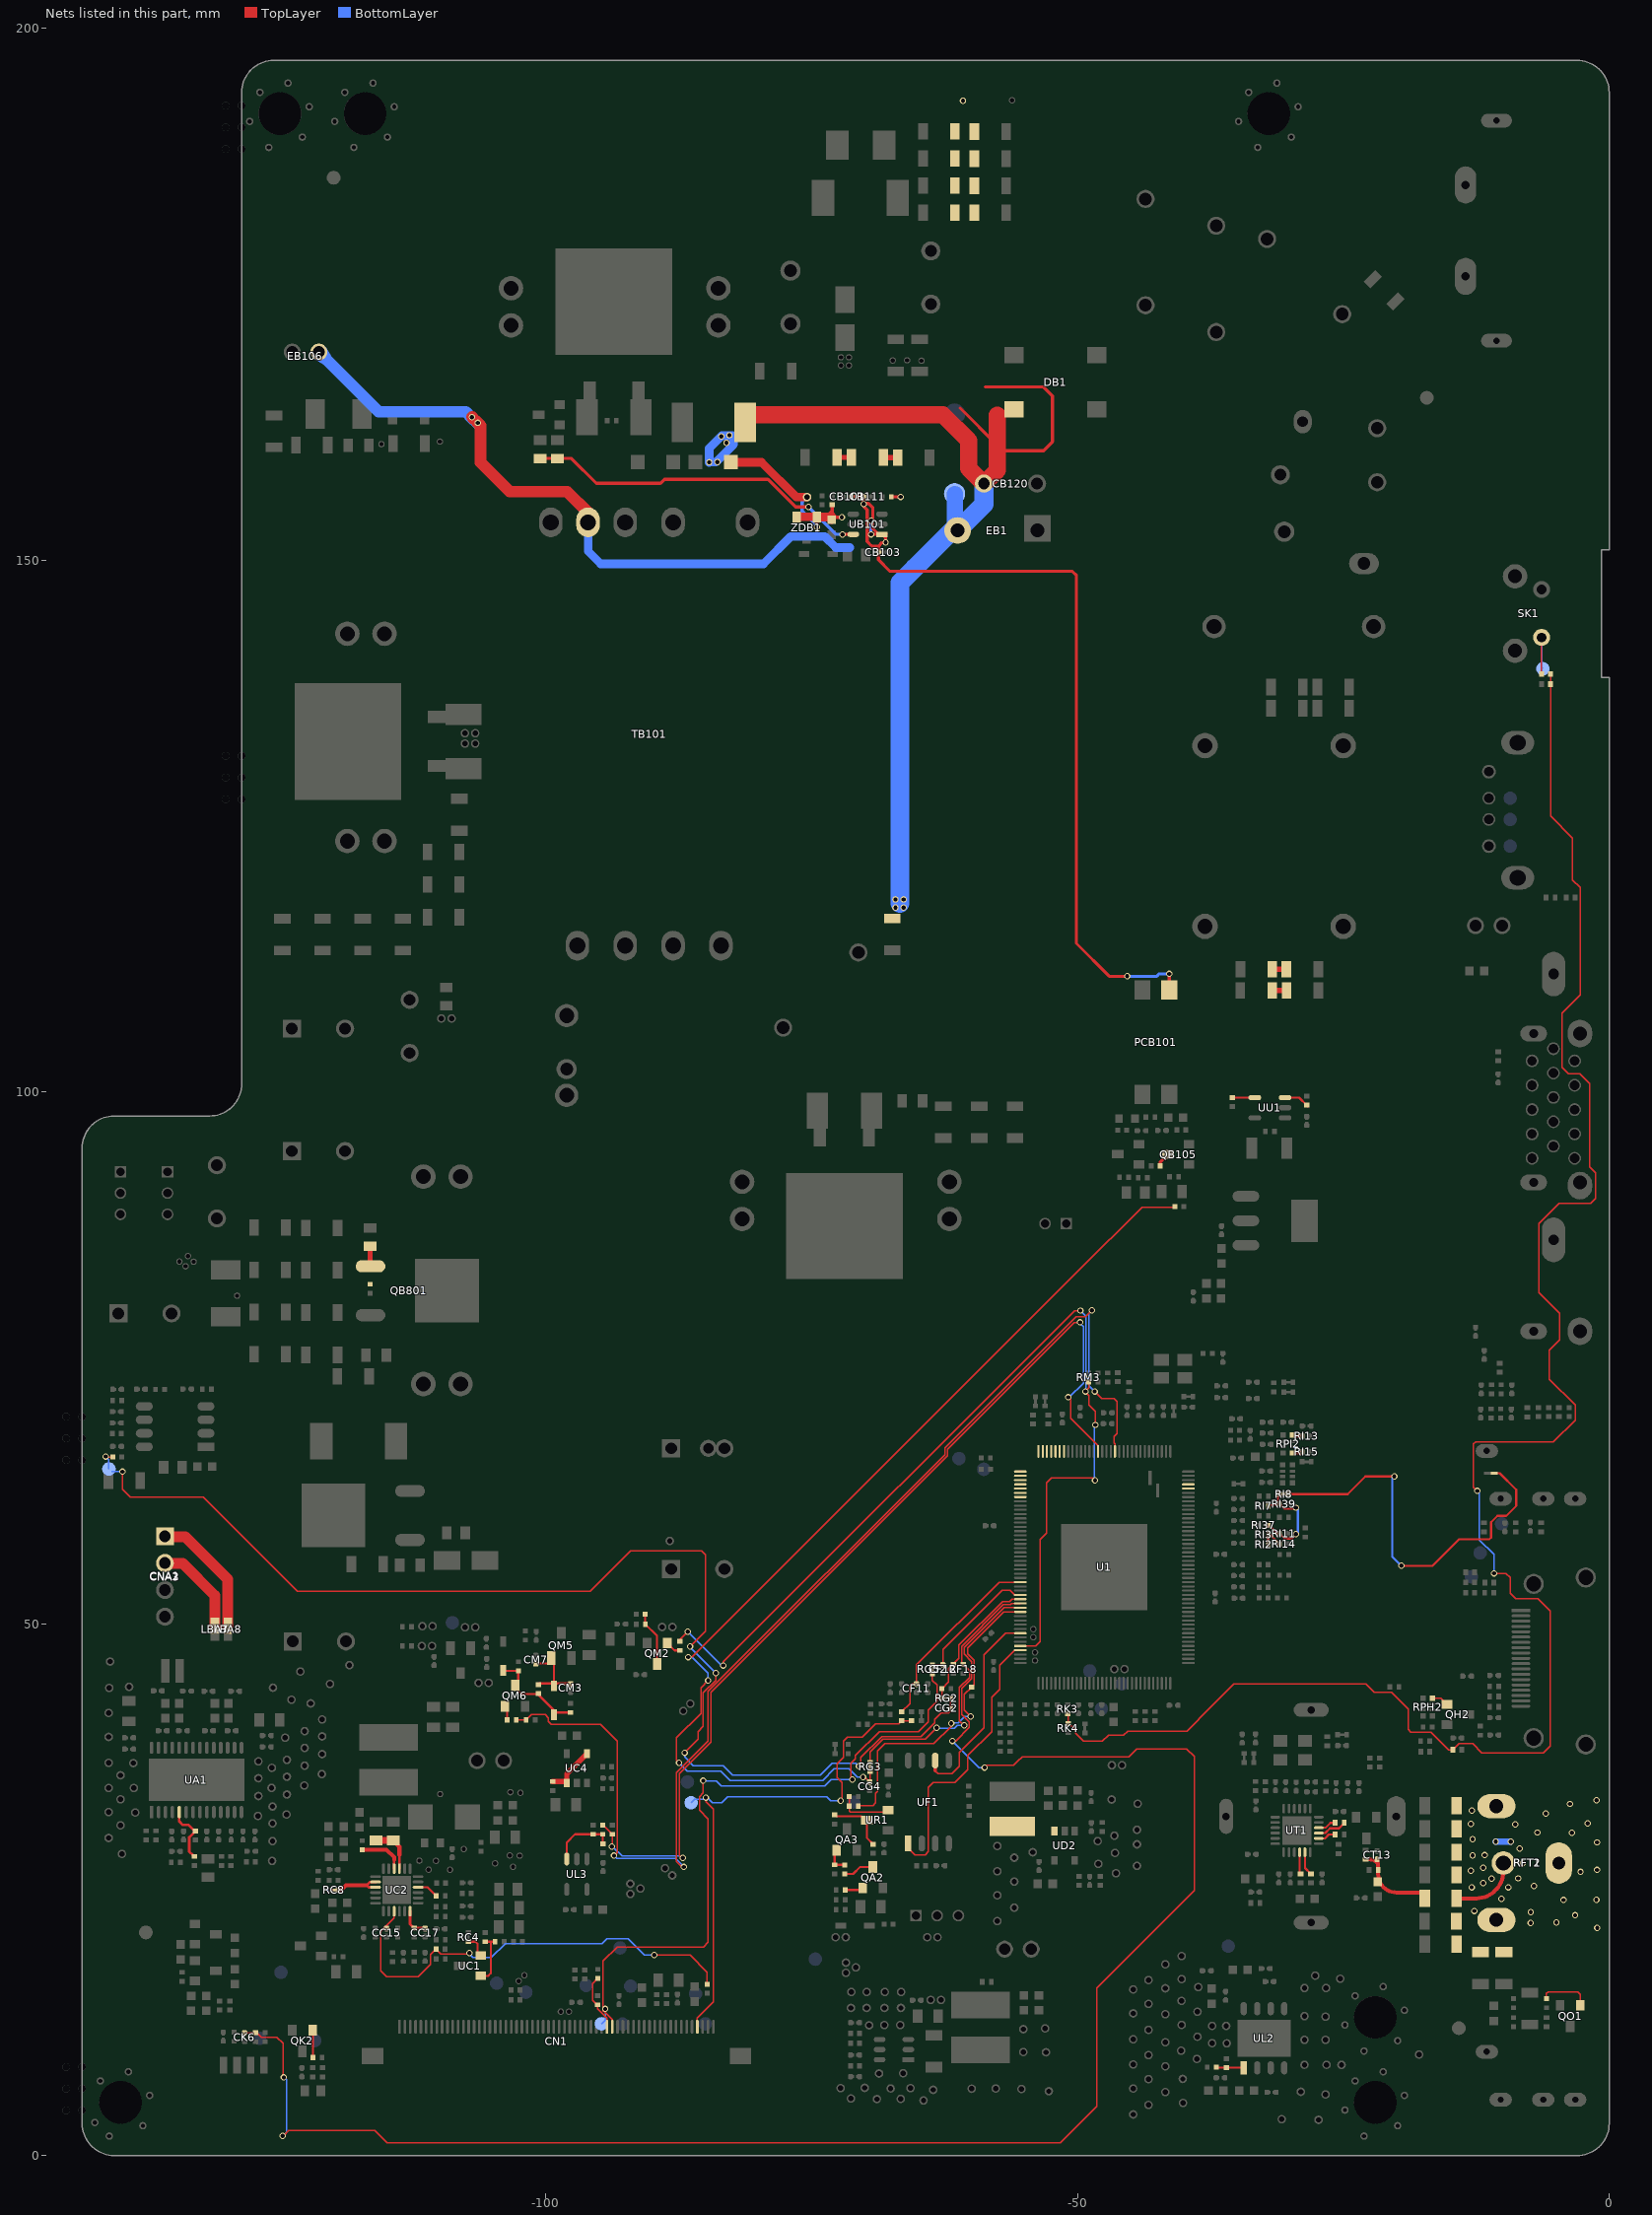
[diagram p0: the nets of this part, all layers, seen from the top]
# Altium PCB MISC86383-9.PcbDoc (part 14 of 18)
Units mm, origin at the board's own origin, x right, y up, seen from the top; angles counter-clockwise.
Board outline 143.6 x 197 mm, 2 copper layers (TopLayer, BottomLayer), stack 1.571 mm thick; 743 components, 401 nets, 2996 pads, 1077 vias.
Unrouted connection lines stored in the file: 4.

## Via types
v1: diameter 0.6, hole 0.4, TopLayer to BottomLayer, tented both sides, 993 vias
v2: diameter 0.6, hole 0.4, TopLayer to BottomLayer, 65 vias
v3: diameter 0.7, hole 0.5, TopLayer to BottomLayer, tented both sides, 15 vias
v4: diameter 0.8, hole 0.5, TopLayer to BottomLayer, tented both sides, 4 vias

## Nets (pads, with @x,y where several pads share a name; then routed paths per layer and width w, separated by ;. In a path a pad name is that pad's centre, name@x,y a point inside that pad or via, vN(x,y) a via of type N, cw(c..) or ccw(c..) an arc to the next point about the centre after c; other vN are vias at no path point) (continued)
NetDK1_K: DK1.K DK2.K RK3.2 RK4.1 RK6.1 | length 177.8
  TopLayer w0.127: RK3.2@-50.862,41.54 -50.862,40.625 RK4.1@-50.874,40.612 -50.779,40.612 -50.189,40.022 -50.189,39.704 -49.439,38.955 -47.656,38.955 -47.092,39.519 -45.657,39.519 -45.281,39.895 -39.723,39.895 -37.47,42.149 -37.47,42.171 -35.277,44.364 -22.893,44.364 -22.069,43.539 -20.456,43.539 -18.91,41.993 -18.91,40.058 -18.676,39.825 -16.762,39.825 -15.088,38.151 DK2.K@-14.7,38.151 -14.13,38.721 -12.813,38.721 -11.969,37.877 -6.175,37.877 -5.537,38.515 -5.537,51.225 -6.687,52.375 -8.81,52.375 -9.301,52.866 -9.301,54.333 -9.708,54.74 v1(-10.825,54.74) ; v1(-12.408,62.497) -12.75,62.839 -12.75,66.897 -12.56,67.087 -5.265,67.087 -3.2,69.152 -3.2,70.561 -5.625,72.986 -5.625,75.732 -4.674,76.683 -4.674,79.18 -6.617,81.123 -6.617,87.624 -4.705,89.535 -1.753,89.535 -1.295,89.992 -1.295,92.411 -1.829,92.945 -1.829,100.787 -2.743,101.702 -3.835,101.702 -4.445,102.311 -4.445,107.417 -2.729,109.132 -2.729,119.219 -3.437,119.927 -3.437,123.888 -5.519,125.969 DK1.K@-5.519,138.354 RK6.1@-5.519,139.294
  BottomLayer w0.127: v1(-12.408,62.497) -12.197,62.286 -12.197,57.897 -10.825,56.525 v1(-10.825,54.74)
NetKEY_1: KEY.1 RK6.2 SK1.2 | length 6.5
  TopLayer w0.127: RK6.2@-6.369,139.294 -6.369,142.731 SK1.2@-6.35,142.75
  BottomLayer w0.127: SK1.2@-6.35,142.75 -6.35,139.916 KEY.1@-6.236,139.802
NetLD2_2: LD2.2 UD2.3
NetLT1_2: LT1.2 UT1.23 | length 2.3
  TopLayer w0.203: UT1.23@-28.61,28.52 -28.61,27.033 LT1.2@-28.064,26.487
NetLT2_1: LT2.1 UT1.22 | length 2
  TopLayer w0.203: LT2.1@-29.11,26.568 UT1.22@-29.11,28.52
NetLT8_1: LT8.1 UT1.2 | length 1.7
  TopLayer w0.203: UT1.2@-27.31,29.82 -26.732,29.82 -26.376,30.177 LT8.1@-25.771,30.177
NetLT10_1: LT10.1 UT1.4 | length 1.7
  TopLayer w0.203: UT1.4@-27.31,30.82 -26.669,30.82 -26.208,31.282 LT10.1@-25.771,31.282
NetLT10_2: LT10.2 UT1.3 | length 2.8
  TopLayer w0.203: UT1.3@-27.31,30.32 -26.702,30.32 -26.261,30.761 -25.41,30.761 -24.921,31.25 LT10.2@-24.921,31.282
NetQA2_B: QA2.B RA19.1 | length 1.7
  TopLayer w0.203: RA19.1@-71.855,24.98 -70.388,24.98 QA2.B@-70.21,25.157
NetQA2_C: QA2.C RA10.1 | length 2.9
  TopLayer w0.203: RA10.1@-71.89,26.472 -71.096,26.472 -70.428,27.139 QA2.C@-69.245,27.139
NetQA3_B: QA3.B RA10.2 RA38.2 | length 2.4
  TopLayer w0.203: QA3.B@-72.649,28.713 -72.83,28.532 RA38.2@-72.83,27.334 -71.903,27.334 RA10.2@-71.89,27.322
NetQB105_C: QB105.C RB180.1 | length 1.4
  TopLayer w0.3: RB180.1@-42.222,93.066 -42.222,93.428 QB105.C@-41.504,94.145
NetQB801_G: QB801.G RB807.2 RB808.2 | length 1.9
  TopLayer w0.5: RB807.2@-116.523,85.494 -116.523,83.657 QB801.G@-116.484,83.618
NetQH2_B: QH2.B RPH2.7 | length 1.6
  TopLayer w0.127: RPH2.7@-16.606,43.014 -15.832,43.014 QH2.B@-15.241,42.423
NetQK2_B: QK2.B RK20.1 | length 2.6
  TopLayer w0.203: QK2.B@-121.933,11.786 -121.888,11.741 RK20.1@-121.888,9.195
NetQM2_B: QM2.B RM4.1 | length 1.7
  TopLayer w0.203: QM2.B@-88.424,48.342 QM2.B@-88.57,48.197 -88.57,48.171 -87.891,47.492 RM4.1@-87.376,47.492
NetQM2_C: QM2.C RM1.1 RM2.1 | length 5.1
  TopLayer w0.203: RM1.1@-90.647,50.902 -90.647,49.975 RM2.1@-90.634,49.962 -89.535,48.863 QM2.C@-89.535,46.215
NetQM6_B: QM6.B RM8.2 | length 1.4
  TopLayer w0.203: QM6.B@-103.848,42.228 -103.625,42.005 RM8.2@-103.625,40.957
NetQO1_B: QO1.B RO10.1 | length 4.9
  TopLayer w0.127: RO10.1@-5.893,14.746 -5.893,15.24 -5.74,15.392 -2.946,15.392 -2.705,15.151 QO1.B@-2.705,14.118
NetRA4_1: RA4.1 RA14.2 UA1.5 | length 5.6
  TopLayer w0.254: UA1.5@-134.47,32.291 -134.47,31.411 -134.14,31.08 -133.592,31.08 -133.02,30.509 RA14.2@-132.947,30.509 -133.53,29.925 -133.53,28.58 -133.173,28.223 -133.048,28.223 RA4.1@-133.004,28.223
NetRB101_2: RB101.2 RB102.1 | length 1.3
  TopLayer w0.5: RB102.1@-31.685,109.563 RB101.2@-30.342,109.563
NetRB106_1: RB106.1 RB107.1 UB101.6 | length 32.7
  TopLayer w0.3: RB107.1@-100.546,159.56 -100.533,159.573 RB106.1@-98.92,159.573 -97.584,159.573 -95.25,157.239 -89.217,157.239 -88.836,157.62 -79.111,157.62 -76.508,155.016 v2(-75.286,155.016) ; v2(-72.098,152.438) -72.095,152.441 UB101.6@-71.086,152.441
  BottomLayer w0.3: v2(-75.286,155.016) -72.707,152.438 v2(-72.098,152.438)
NetRB141_1: RB141.1 RB142.2 | length 1.9
  TopLayer w0.3: RB142.2@-31.672,111.544 -31.067,111.544
  TopLayer w0.5: RB142.2@-31.672,111.544 -31.66,111.557 RB141.1@-30.354,111.557
NetRB143_1: RB143.1 RB144.2 | length 1.3
  TopLayer w0.5: RB144.2@-68.261,159.677 -68.248,159.664 RB143.1@-66.918,159.664
NetRB144_1: RB144.1 RB145.2 | length 1.4
  TopLayer w0.5: RB145.2@-72.617,159.677 RB144.1@-71.261,159.677
NetRB150_1: pad.VIA5@-60.769,193.218 RB150.1 RB151.1 RB152.1 RB153.2 RB154.2 RB155.2 RB156.1 RB157.2
NetRC2_1: RC2.1 RC3.2 UC1.1 | length 4.9
  TopLayer w0.203: UC1.1@-106.121,16.891 -105.41,16.891 -105.177,17.124 -105.177,20.013 ; RC3.2@-105.715,20.098 -104.787,20.098 RC2.1@-104.768,20.117
NetRC4_1: RC4.1 UC1.2 | length 2.2
  TopLayer w0.203: RC4.1@-107.29,20.098 -106.611,20.098 -106.426,19.914 -106.426,19.05 -106.172,18.796 UC1.2@-106.121,18.796
NetRC8_2: RC8.2 RC8.3 UC2.2 UC2.3 | length 4.7
  TopLayer w0.254: UC2.3@-116.014,25.223 -116.638,25.223 -116.827,25.413 -116.517,25.723 UC2.2@-116.014,25.723
  TopLayer w0.381: RC8.2@-119.52,24.948 -119.269,24.948 -118.804,25.413 -116.827,25.413
NetRC13_1: RC13.1 UC2.16 | length 2
  TopLayer w0.203: UC2.16@-112.014,25.223 -111.131,25.223 RC13.1@-110.309,24.401
NetRC36_1: RC36.1 UC4.1 UC4.4 | length 4.9
  TopLayer w0.508: RC36.1@-99.365,35.172 -98.165,35.172 UC4.1@-98.029,35.036 -98.029,35.886 UC4.4@-96.129,37.786
NetRG6_1: RG6.1 UC2.22 | length 4.4
  TopLayer w0.254: UC2.22@-114.264,26.973 -114.264,27.813
  TopLayer w0.381: RG6.1@-117.259,28.76 -114.98,28.76 -114.264,28.044 -114.264,27.813
NetRG58_1: RG58.1 RG63.1 UC2.21 | length 4.5
  TopLayer w0.254: UC2.21@-113.764,26.973 -113.764,28.27
  TopLayer w0.381: RG63.1@-114.351,29.627 -113.764,29.04 -113.764,28.27
  TopLayer w0.61: RG58.1@-115.976,29.627 RG63.1@-114.351,29.627
NetRI2_1: RI2.1 RI3.2 RI14.2 | length 2.3
  TopLayer w0.178: RI14.2@-30.991,57.495 RI14.2@-30.989,57.497
  TopLayer w0.203: RI2.1@-32.057,57.483 RI3.2@-32.057,58.372 -31.867,58.372 RI14.2@-30.991,57.495
NetRI7_2: RI7.2 RI8.1 RI11.2 RI37.2 RI39.2 | length 9.7
  TopLayer w0.178: RI7.2@-32.057,61.077 -31.968,61.166 RI39.2@-31.015,61.166 ; RI8.1@-31.015,62.194 -31.136,62.074 -31.136,61.414 RI39.2@-31.002,61.28 -30.995,61.28 -30.529,60.814 v1@-29.57,60.814
  TopLayer w0.203: RI37.2@-32.057,59.248 -31.974,59.248 -31.136,58.41 RI11.2@-31.002,58.41 ; RI11.2@-31.002,58.486 -30.523,58.007 -29.832,58.007 -29.472,58.368 v1(-29.472,58.422)
  BottomLayer w0.203: v1(-29.472,58.422) -29.274,58.621 -29.274,60.713 v1(-29.472,60.912)
NetRI8_2: RI8.2 RI8.3 RI10.JP_2K | length 37.7
  TopLayer w0.203: RI8.2@-30.165,62.194 -24.591,62.194 -22.935,63.851 v1(-20.206,63.851) ; v1(-19.553,55.452) -16.634,55.452 -14.149,57.937 -11.29,57.937 -11.112,58.115 -11.112,59.538 -10.506,60.144 -9.68,60.144 -8.737,61.087 -8.737,62.597 -10.3,64.16 RI10.JP_2K@-10.793,64.16
  BottomLayer w0.203: v1(-20.206,63.851) -20.404,63.652 -20.404,56.303 v1(-19.553,55.452)
NetRI13_2: RI13.2 RPI2.2 | length 1
  TopLayer w0.305: RPI2.2@-29.771,67.756 -29.671,67.655 RI13.2@-28.868,67.655 RI13.2@-28.907,67.616
NetRI15_2: RI15.2 RPI2.8 | length 1
  TopLayer w0.254: RPI2.8@-29.771,66.056 -28.994,66.056 RI15.2@-28.868,66.182
NetRL3_2: RL3.2 RL50.2 RL51.2 UL3.3 | length 6.2
  TopLayer w0.203: UL3.3@-98.016,27.879 -98.016,29.441 -97.25,30.207 RL3.2@-95.555,30.207 RL51.2@-94.64,30.207 -94.64,29.33 RL50.2@-94.628,29.318
NetRL4_2: RL4.2 RL5.1 UL2.1 | length 3.1
  TopLayer w0.203: RL5.1@-36.945,8.306 -36.901,8.262 RL4.2@-35.992,8.262 -34.387,8.262 UL2.1@-34.366,8.241 UL2.1@-34.366,7.849 ; UL2.1@-34.461,7.754 UL2.1@-34.385,7.83
NetRR5_1: RR5.1 RR6.1 UR1.3 | length 5.8
  TopLayer w0.203: RR6.1@-72.847,32.099 -72.809,32.061 -72.651,31.902 -70.333,31.902 -69.963,31.533 UR1.3@-69.792,31.533 -69.792,29.85 RR5.1@-69.207,29.265
NetRU4_1: RU4.1 UU1.4 | length 2.1
  TopLayer w0.203: RU4.1@-35.425,99.477 UU1.4@-33.327,99.477
NetRU45_1: RU45.1 UU1.3 | length 2.5
  TopLayer w0.203: UU1.3@-30.477,99.477 -29.164,99.477 -28.448,98.762 RU45.1@-28.346,98.66
OE1: CN1.57 OE1.1 RG40.2 RG46.2 | length 50.6
  TopLayer w0.127: CN1.57@-85.75,12.103 -85.75,12.923 -84.226,14.448 -84.226,32.564 -84.95,33.289 v1(-84.95,33.655) v1@-84.811,33.655 ; v1(-72.263,33.363) -72.128,33.498 -72.128,35.082 -72.606,35.56 -72.606,36.852 -72.005,37.453 -72.005,38.956 -71.642,39.319 -70.244,39.319 -68.982,40.581 -66.817,40.581 RG46.2@-66.523,40.875 RG40.2@-65.608,40.875
  BottomLayer w0.127: OE1.1@-86.335,33.172 -85.992,33.515 -85.09,33.515 v1(-84.95,33.655) ; v1@-84.811,33.655 -84.315,33.16 -83.455,33.16 -82.897,33.718 -73.566,33.718 -73.219,33.371 -72.271,33.371 v1(-72.263,33.363)
OE1/: CF11.1 RG46.1 U1.105 | length 18.2
  TopLayer w0.127: RG46.1@-66.523,41.725 -65.735,42.513 -65.735,44.145 -65.514,44.367 CF11.1@-65.151,44.367 -65.151,46.141 -57.379,53.913 U1.105@-55.371,53.913
PAIRMODE/: CN1.40 RG7.1 RG12.2 | length 5.4
  TopLayer w0.127: RG12.2@-95.123,14.174 RG12.2@-95.123,14.122 ; RG7.1@-95.11,16.656 -95.593,16.174 -95.593,14.592 -95.149,14.148 RG12.2@-95.123,14.122 ; CN1.40@-94.25,12.103 -94.25,12.916 -95.123,13.789 RG12.2@-95.123,14.122
PANEL5V_MOS_G: CM3.1 CM7.1 DM1.K QM5.G RM7.2 | length 7.3
  TopLayer w0.203: CM7.1@-100.94,46.197 -100.87,46.266 QM5.G@-99.682,46.266 ; RM7.2@-100.711,44.278 -100.602,44.388 DM1.K@-99.225,44.388 ; QM5.G@-99.49,46.781 -99.225,46.516 DM1.K@-99.225,44.388 ; DM1.K@-99.225,44.149 DM1.K@-99.225,44.388 ; CM3.1@-97.522,44.388 CM3.1@-97.665,44.388 DM1.K@-99.225,44.388
PANEL_DVDD_EN_IC: RL7.2 RL51.1 U1.64 | length 90.4
  TopLayer w0.127: RL51.1@-94.64,31.057 -94.576,31.057 RL7.2@-93.726,30.207 -93.726,29.108 v1(-93.777,29.058) ; v1(-87.109,27.991) -87.109,27.864 -87.173,27.927 -87.447,28.202 -87.447,35.892 -84.48,38.859 -84.48,43.568 -62.225,65.824 -62.225,66.419 -50.323,78.321 -49.797,78.321 v1(-49.771,78.346) ; v1(-50.876,71.298) -50.622,71.298 -50.619,71.295 -50.619,69.33 -48.071,66.782 U1.64@-48.071,66.213
  BottomLayer w0.127: v1(-93.777,29.058) -93.726,29.007 -93.675,29.007 -92.837,28.169 -87.287,28.169 v1(-87.109,27.991) ; v1(-50.876,71.298) -50.767,71.298 -49.451,72.613 -49.451,77.925 -49.771,78.245 v1(-49.771,78.346)
PANEL_ON: DM1.A DM3.A QM6.C RM5.1 RM7.1 RM12.1 | length 10.1
  TopLayer w0.203: DM3.A@-104.136,45.555 -104.026,45.665 -103.988,45.704 -103.949,45.665 -103.852,45.568 RM12.1@-102.572,45.568 ; RM12.1@-102.565,45.574 RM12.1@-102.572,45.568 ; RM5.1@-97.665,41.658 -99.016,41.658 DM1.A@-99.225,41.449 -99.225,41.859 -100.711,43.345 RM7.1@-100.711,43.428 -100.756,43.383 -102.26,43.383 -102.883,44.005 QM6.C@-102.883,44.21 -102.591,44.502 -102.591,45.549 RM12.1@-102.572,45.568
PANEL_ON/OFF: RM8.1 RM10.1 U1.60 | length 113.7
  TopLayer w0.127: RM8.1@-102.775,40.957 RM10.1@-101.847,40.957 -101.339,41.465 -100.063,41.465 -99.746,41.148 -99.746,40.805 -99.498,40.557 -94.875,40.557 -93.269,38.951 -93.269,28.511 v1(-93.586,28.194) ; v1(-87.008,27.127) -87.097,27.038 -87.701,27.643 -87.701,35.997 -84.734,38.965 -84.734,43.638 -62.479,65.893 -62.479,66.525 -50.236,78.767 -50.124,78.88 -49.251,78.88 v1(-48.654,79.477) ; v1(-48.385,71.848) -47.704,71.167 -46.574,71.167 -46.286,70.879 -46.286,67.894 -46.561,67.619 -46.561,67.468 -46.561,67.023 -46.468,66.93 -46.468,66.216 U1.60@-46.471,66.213
  BottomLayer w0.127: v1(-93.586,28.194) -93.307,27.915 -87.795,27.915 v1(-87.008,27.127) ; v1(-48.654,79.477) -48.943,79.187 -48.943,72.406 v1(-48.385,71.848)
PC_LIN: U1.43
PC_RIN: U1.42
POL: CN1.41 POL.1 RG52.2 RG52.3 | length 65.2
  TopLayer w0.127: CN1.41@-93.75,12.103 -93.75,12.775 -94.412,13.437 ; v1(-85.192,35.242) -85.192,34.107 -85.555,33.744 -85.555,32.482 -84.734,31.661 -84.734,20.037 -85.167,19.604 -93.29,19.604 -94.602,18.292 v1@-94.602,13.779 ; v1(-71.158,35.344) -71.309,35.495 -71.309,36.892 -70.879,37.322 -70.879,37.611 -68.629,39.86 -64.946,39.86 -64.018,40.789 -64.018,41.887 -63.195,42.709 -63.195,44.247 -63.64,44.691 RG52.2@-63.64,45.295 ; v1@-94.602,13.779 -94.602,13.627 -94.412,13.437 ; v1@-94.602,13.779 -94.513,13.691 -94.501,13.691 v1(-94.412,13.779) -94.412,13.437
  BottomLayer w0.127: POL.1@-94.767,12.383 -94.412,12.738 v1(-94.412,13.779) ; v1(-85.192,35.242) -84.963,35.242 -84.933,35.212 -83.98,35.212 -83.502,34.734 -73.777,34.734 -73.159,35.352 -71.166,35.352 v1(-71.158,35.344)
POL/: CF12.1 RG52.1 U1.108 | length 12.3
  TopLayer w0.127: RG52.1@-63.779,46.126 RG52.1@-63.7,46.206 ; RG52.1@-63.64,46.145 -62.674,46.145 CF12.1@-62.649,46.17 -62.649,47.565 -57.064,53.151 -56.358,53.151 -55.92,52.713 U1.108@-55.371,52.713
POW_EN: RM3.2 RM4.2 U1.120 | length 93.3
  TopLayer w0.127: RM4.2@-87.376,48.342 -87.376,48.514 v1(-86.639,49.251) ; v1(-83.299,46.076) -83.299,46.423 -50.271,79.451 v1(-49.733,79.451) ; U1.120@-55.371,47.913 -53.935,47.913 -53.511,48.336 -53.511,57.926 -52.929,58.508 -52.929,59.021 -52.929,63.232 -52.436,63.725 -48.593,63.725 v1(-48.347,63.479) ; RM3.2@-48.944,72.845 -48.944,72.731 -48.944,72.198 -49.262,71.88 v1(-49.262,71.842) -49.262,71.785 -48.926,71.45 -48.926,70.599 -48.322,69.994 v1(-48.322,68.698)
  BottomLayer w0.127: v1(-86.639,49.251) -83.49,46.101 -83.325,46.101 v1(-83.299,46.076) ; v1(-49.733,79.451) -49.197,78.915 -49.197,71.906 v1(-49.262,71.842) ; v1(-48.347,63.479) -48.401,63.533 -48.401,68.619 v1(-48.322,68.698)
PS_ON: CG4.1 RB182.2 RG3.2 RG3.3 | length 96.2
  TopLayer w0.127: v1(-87.465,36.932) -87.701,37.168 -87.701,39.299 -85.42,41.58 -85.42,43.981 v1(-84.734,44.666) ; v1(-86.601,46.863) -86.601,46.888 -86.212,46.888 -49.94,83.16 -49.936,83.16 -43.927,89.169 RB182.2@-40.898,89.169 ; v1(-70.167,35.585) -70.129,35.547 -69.946,35.547 CG4.1@-69.545,35.147 -69.52,35.172 RG3.2@-69.52,36.126 ; RB182.2@-40.898,89.169 -40.836,89.169 RB182.2@-40.836,89.23 RB182.2@-40.898,89.169
  BottomLayer w0.127: v1(-87.465,36.932) -86.677,36.144 -83.525,36.144 -82.653,35.273 -73.957,35.273 -72.874,36.355 -71.476,36.355 -70.706,35.585 v1(-70.167,35.585) ; v1(-86.601,46.863) -86.24,46.863 -84.734,45.357 v1(-84.734,44.666)
PWM0: RF13.1 RF14.2 RG2.1 U1.109 | length 13.1
  TopLayer w0.127: RG2.1@-62.757,43.079 RF14.2@-62.757,43.901 -62.141,44.517 -62.141,45.783 -61.715,46.21 -61.153,46.772 -61.153,47.984 -57.037,52.1 -56.365,52.1 -56.152,52.313 U1.109@-55.371,52.313
PWM1: RF18.1 RG3.1 U1.110 | length 26.4
  TopLayer w0.127: RG3.1@-69.52,36.976 -69.52,37.964 -68.309,39.175 -64.308,39.175 -63.246,40.236 v1(-63.232,40.222) ; v1(-60.655,40.437) -61.1,40.881 -61.1,43.999 -60.16,44.938 -60.16,45.573 RF18.1@-60.754,46.168 -60.899,46.312 -60.899,47.879 -56.983,51.795 -56.311,51.795 -56.193,51.913 U1.110@-55.371,51.913
  BottomLayer w0.127: v1(-63.232,40.222) -63.194,40.184 -61.568,40.184 -61.316,40.437 v1(-60.655,40.437)
PWM_REF: CG2.1 PWM_REF.1 RB813.2 RG2.2 RG2.3 | length 117.4
  TopLayer w0.127: v2(-141.396,65.731) -141.35,65.684 RB813.2@-140.719,65.684 ; v2(-139.802,64.3) -139.802,62.662 -139.065,61.925 -132.205,61.925 -123.341,53.061 -95.809,53.061 -92.024,56.845 -85.369,56.845 -85.001,56.477 -85.001,49.289 v1(-86.436,47.854) ; v1@-86.957,37.859 -86.963,37.865 -85.681,39.148 -85.681,39.859 -85.191,40.348 -85.191,43.504 -84.01,44.684 v1(-84.01,45.352) v1@-84.061,45.402 ; v1(-70.551,36.591) -70.371,36.771 -70.371,37.436 -68.404,39.403 -64.708,39.403 -63.435,40.676 -63.435,40.996 -62.843,41.588 -62.146,41.588 -61.932,41.801 -61.932,42.05 -61.932,43.053 RG2.2@-61.907,43.078
  BottomLayer w0.127: v2@-141.402,65.725 v2(-141.396,65.731) -141.084,65.419 PWM_REF.1@-141.084,64.554 ; PWM_REF.1@-140.83,64.3 v2(-139.802,64.3) ; v1(-86.944,37.871) -86.944,37.464 -86.133,36.652 -83.314,36.652 -82.443,35.781 -74.167,35.781 -73.085,36.863 -70.823,36.863 v1(-70.551,36.591) ; v1(-86.436,47.854) -86.436,47.777 v1(-84.01,45.352)
REF: CC17.2@-111.36,21.38 CC17.2@-111.36,21.205 RG22.1 UC2.12 | length 2.8
  TopLayer w0.254: UC2.12@-112.764,22.973 -112.764,21.768 RG22.1@-112.376,21.38 CC17.2@-111.36,21.38
REMOTE: CK6.2@-128.321,11.55 CK6.2@-128.321,11.375 RK16.1 U1.111 | length 170.9
  TopLayer w0.127: CK6.2@-128.321,11.55 -127.305,11.55 -127.171,11.55 -126.737,11.116 -125.289,11.116 -124.717,10.544 -124.717,7.42 v1(-124.638,7.341) ; v1(-124.739,1.841) -124.676,1.841 -124.168,2.349 -116.075,2.349 -114.898,1.173 -51.612,1.173 -48.176,4.608 -48.176,15.759 -39.008,24.927 -39.008,37.516 -39.736,38.244 -44.415,38.244 -45.151,37.507 -55.2,37.507 -55.636,37.071 -55.639,37.071 -56.032,36.678 -58.73,36.678 -58.801,36.678 -58.73,36.606 v1(-58.73,36.483) ; v1(-61.773,38.989) -61.436,38.989 -60.173,40.252 -60.173,40.754 -60.871,41.453 -60.871,43.904 -59.931,44.844 -59.931,46.444 -60.645,47.157 -60.645,47.774 -56.906,51.513 U1.111@-55.371,51.513
  BottomLayer w0.127: v1(-124.739,1.841) -124.392,2.189 -124.392,7.145 -124.612,7.366 v1(-124.638,7.341) ; v1(-61.773,38.989) -59.267,36.483 v1(-58.73,36.483)
RESET_H: DR1.K RR1.1 U1.112 | length 30.7
  TopLayer w0.127: RR1.1@-70.619,32.842 -70.543,32.918 -69.215,32.918 -68.979,33.155 -68.979,34.05 -68.802,34.227 -68.802,38.035 -68.12,38.717 -63.509,38.717 -61.87,40.357 v1(-61.87,40.649) ; v1(-60.046,41.288) -60.642,41.885 -60.642,43.351 DR1.K@-59.957,44.037 -59.703,44.291 -59.703,46.545 -60.345,47.188 -60.345,47.714 -56.946,51.113 U1.112@-55.371,51.113
  BottomLayer w0.127: v1(-61.87,40.649) -61.853,40.665 -61.201,40.665 -60.592,41.275 -60.058,41.275 v1(-60.046,41.288)
RESET_H/: RR1.2 RR2.1 UR1.2 | length 5.1
  TopLayer w0.127: RR2.1@-71.469,33.757 RR1.2@-71.469,32.842 -71.469,32.404 -71.374,32.309 -67.986,32.309 UR1.2@-67.81,32.485
RF_IN: CT40.1 RFT1.1 RFT2.1 | length 6.9
  TopLayer w0.368: CT40.1@-14.349,23.786 cw(c-13.955,23.786) -13.955,24.181 -12.49,24.181 ccw(c-12.49,26.721) -9.95,26.721 RFT2.1@-9.95,27.5
RF_INPUT: CT13.1 CT40.2 LT3.1 LT9.1 LT11.1 | length 7.9
  TopLayer w0.368: LT3.1@-22.907,27.847 -22.536,27.847 cw(c-22.536,26.84) -21.823,27.552 cw(c-22.001,27.375) -21.75,27.375 -21.75,26.838 -21.75,26.81 cw(c-21.721,26.81) LT11.1@-21.721,26.838 -21.721,26.445 ccw(c-20.004,26.445) -20.004,24.727 CT40.2@-17.361,24.727 ; CT40.2@-17.463,23.673 ccw(c-17.463,23.786) CT40.2@-17.349,23.786
RFGND: CT41.2 CT42.2 CT43.2 CT44.2 CT45.2 CT46.2 CT47.2 CT48.2 RFT1.2 RFT1.3 RFT1.4 RFT2.2 RFT2.3 RFT2.4 | length 1.4
  BottomLayer w0.61: v1(-10.664,29.513) -9.271,29.513 v1(-9.259,29.524)
  other v1: -1.12,21.392 -7.375,21.859 -4.963,21.922 -3.202,22.586 -7.373,22.895 -12.679,22.997 -4.282,24.023 -1.205,24.039 -10.123,24.137 -12.932,25.219 -9.478,25.219 -7.064,25.335 -11.85,25.633 -11.067,26.025 -8.569,26.059 -2.694,26.671 -13,26.765 -1.132,26.849 -11.838,27.061 -8.12,27.463 -12.843,28.205 -11.711,28.246 -8.431,28.868 -1.132,29.444 -12.843,29.739 -3.511,30.34 -6.755,30.371 -8.825,31.143 -13,31.179 -2.008,31.22 -5.952,32.163 -12.906,32.432 -3.696,33.059 -1.194,33.399
RML_0N_IC: U1.79 | length 0
  TopLayer w0.155: U1.79@-55.393,64.335 U1.79@-55.371,64.313
RML_1N_IC: U1.81
RML_1P_IC: U1.80
RML_2N_IC: U1.83
RML_2P_IC: U1.82
RML_CKN_IC: U1.85
RML_CKP_IC: U1.84
ROUT+: CNA1.1 CNA2.1 CNA3.1 LBA8.2 LBA8.3 | length 12.1
  TopLayer w1.016: CNA3.1@-135.814,58.195 -133.887,58.195 -129.899,54.207 LBA8.3@-129.899,49.692
ROUT-: CNA1.2 CNA2.2 CNA3.2 LBA7.2 LBA7.3 | length 8.9
  TopLayer w1.016: CNA3.2@-135.814,55.675 -134.148,55.675 -131.118,52.644 LBA7.3@-131.118,49.692
RST: CC15.1 RC10.1 RG41.1 UC2.9 | length 42.4
  TopLayer w0.127: CC15.1@-114.98,21.38 CC15.1@-114.98,21.571 ; UC2.9@-114.264,22.973 -114.264,22.325 -115.094,21.495 -115.504,21.085 -115.504,17.359 -114.972,16.828 -111.999,16.828 -110.833,17.994 -110.833,18.878 RC10.1@-110.318,19.393 -109.878,18.952 v1@-107.192,18.952 ; v1(-89.789,18.86) -89.789,18.834 -86.436,18.834 -84.823,17.221 RG41.1@-84.823,16.097
  BottomLayer w0.127: v1(-107.188,19.025) -107.192,19.021 -107.192,18.952 -106.845,18.605 -105.141,18.605 -103.82,19.926 -94.699,19.926 -94.242,20.383 -92.246,20.383 -90.722,18.86 v1(-89.789,18.86)
RXE2_P: U1.78
RXE3_N: U1.75
RXE3_P: U1.74
RXE4_N: U1.73
RXE4_P: U1.72
RXEC_N: U1.77
RXEC_P: U1.76
SGND: CB101.2@-71.216,155.994 CB101.2@-71.391,155.994 CB102.2 CB103.2@-68.538,150.774 CB103.2@-68.713,150.774 CB111.2@-69.986,155.994 CB111.2@-70.161,155.994 CB120.1 DB1.4 DB110.K EB1.2 EB106.2 pad.VIA5@-66.357,117.348 pad.VIA5@-66.357,118.11 pad.VIA5@-67.119,117.348 pad.VIA5@-67.119,118.11 pad.VIA5@-75.425,155.943 pad.VIA5@-82.74,161.76 pad.VIA5@-83.007,161.049 pad.VIA5@-83.49,161.658 pad.VIA5@-83.858,159.245 pad.VIA5@-84.633,159.22 pad.VIA5@-106.94,163.468 pad.VIA5@-106.402,162.929 PCB101.3 RB103.1 RB104.1 RB130.1 RB148.1 TB101.5 TP-TDT.2 UB101.1 ZDB1.1 ZDB1.3 | length 284.3
  TopLayer w0.3: v2(-74.511,153.124) ZDB1.1@-74.511,154.076 -74.252,153.818 CB102.2@-73.114,153.818 CB102.2@-73.076,153.856 ; -73.647,154.076 -73.51,154.214 -73.076,154.648 ; RB103.1@-73.076,155.226 -73.076,154.648 ; v2(-72.161,154.051) -72.682,154.051 ; CB101.2@-71.216,155.994 CB111.2@-70.161,155.994 v2@-70.161,155.341 ; v2(-69.421,152.441) UB101.1@-68.722,152.441 ; v2@-69.238,153.619 -69.238,153.289 ; UB101.1@-68.008,152.463 -68.041,152.431 -68.041,152.095 ; RB104.1@-67.507,155.969 v2(-66.637,155.969) ; -61.036,164.313 -57.549,160.826 -57.037,160.313 -53.188,160.313 -52.348,161.153 -52.348,165.456 -53.194,166.301 -58.687,166.301 ; v2(-45.326,110.884) -47.005,110.884 -50.104,113.982 -50.104,142.596 -50.102,142.598 -50.102,148.576 -50.497,148.972 -67.641,148.972 -68.713,150.044 CB103.2@-68.713,150.774 -68.713,151.327 ; PCB101.3@-41.364,109.586 v2(-41.364,111.112) ; CB102.2@-73.076,153.856 -73.076,154.445 ; CB102.2@-73.076,153.856 -72.881,154.051 -72.682,154.051 ; -73.076,154.445 -73.076,154.648 ; -73.076,154.445 -72.781,154.15 -72.682,154.051 ; v2@-70.161,155.341 v2(-70.112,155.292) -70.112,155.08 -69.781,154.749 -69.781,153.731 -69.781,152.441 -69.781,151.772 -69.394,151.385 -69.336,151.385 -69.278,151.327 -68.713,151.327 ; v2@-70.161,155.341 -70.112,155.341 -69.659,155.341 -69.238,154.92 -69.238,153.731 -69.238,153.289 ; -69.238,153.289 -69.238,152.957 UB101.1@-68.722,152.441 ; UB101.1@-68.722,152.441 UB101.1@-68.386,152.441 -68.041,152.095 ; -68.713,151.327 -68.37,151.67 v2(-68.041,151.67) -68.041,152.095
  TopLayer w0.8: TB101.5@-96.028,153.567 TB101.5@-96.028,154.397 ; DB110.K@-82.59,159.22 -79.718,159.22 -76.441,155.943 pad.VIA5@-75.425,155.943 ; ZDB1.3@-76.416,154.076 ZDB1.1@-74.511,154.076 -73.647,154.076 -73.373,154.076 CB102.2@-73.114,153.818
  TopLayer w1.1: pad.VIA5@-106.94,163.468 pad.VIA5@-106.402,162.929 -106.134,162.662 -106.134,161.049 ; -106.134,162.598 -106.134,161.049 ; TB101.5@-96.028,153.567 -96.028,154.486 -97.993,156.451 -103.391,156.451 -106.134,159.194 -106.134,161.049
  TopLayer w1.6: RB148.1@-81.251,162.979 -80.54,163.69 -62.662,163.69 -60.236,161.265 -60.236,158.65 CB120.1@-58.799,157.213 -57.549,158.463 -57.549,160.826 -57.549,163.645
  BottomLayer w0.3: pad.VIA5@-75.425,155.943 -75.895,155.473 -75.895,154.648 -74.511,153.264 v2(-74.511,153.124) -74.524,153.124 -74.524,152.271 -74.498,152.246 ; v2@-70.112,155.24 v2(-70.112,155.292) ; v2(-69.421,152.441) v2(-69.421,153.731) ; v2(-45.326,110.884) -42.545,110.884 -42.316,111.112 v2(-41.364,111.112)
  BottomLayer w0.8: TB101.5@-96.028,153.567 -96.028,150.867 -94.829,149.667 -79.537,149.667 -76.958,152.246 -74.498,152.246 -73.773,152.246 -72.72,151.193 -71.399,151.193 ; pad.VIA5@-84.633,159.22 -84.633,160.528 -83.496,161.665 -83.439,161.722 -83.007,161.722 -82.74,161.722 -82.461,161.722 -82.334,161.595 -82.334,161.049 -82.334,160.902 -82.597,160.639 pad.VIA5@-83.925,159.312 ; pad.VIA5@-84.595,159.233 pad.VIA5@-84.004,159.233
  BottomLayer w1.1: EB106.2@-121.343,169.583 -119.787,168.027 -115.73,163.97 -107.518,163.97 -106.978,163.43 pad.VIA5@-106.44,162.891
  BottomLayer w1.5: TP-TDT.2@-61.535,156.235 -61.535,153.061 EB1.2@-61.275,152.801
  BottomLayer w1.8: -66.7,117.767 -66.7,118.11 -66.7,147.884 ; -65.325,149.259 -66.7,147.884 ; CB120.1@-58.799,157.213 -58.799,155.276 EB1.2@-61.275,152.801 -61.784,152.801 -66.7,147.884
SPI_CSN: U1.121 UF1.1 | length 26.8
  TopLayer w0.127: UF1.1@-65.916,29.342 -65.916,28.898 -65.281,28.263 -64.316,28.263 -64.011,28.568 -64.011,34.63 -63.551,35.09 -61.542,35.09 -60.338,36.295 -60.338,37.608 -58.077,39.869 -58.077,43.088 -57.313,43.852 -57.313,46.112 -55.916,47.508 -55.916,47.513 U1.121@-55.371,47.513
SPI_SCK: U1.117 UF1.6 | length 19.3
  TopLayer w0.127: -63.376,36.16 -63.106,35.89 -61.82,35.89 -61.1,36.61 -61.1,37.924 -58.788,40.235 -58.788,47.067 -56.743,49.113 U1.117@-55.371,49.113
  TopLayer w0.305: -63.376,36.16 UF1.6@-63.376,37.142